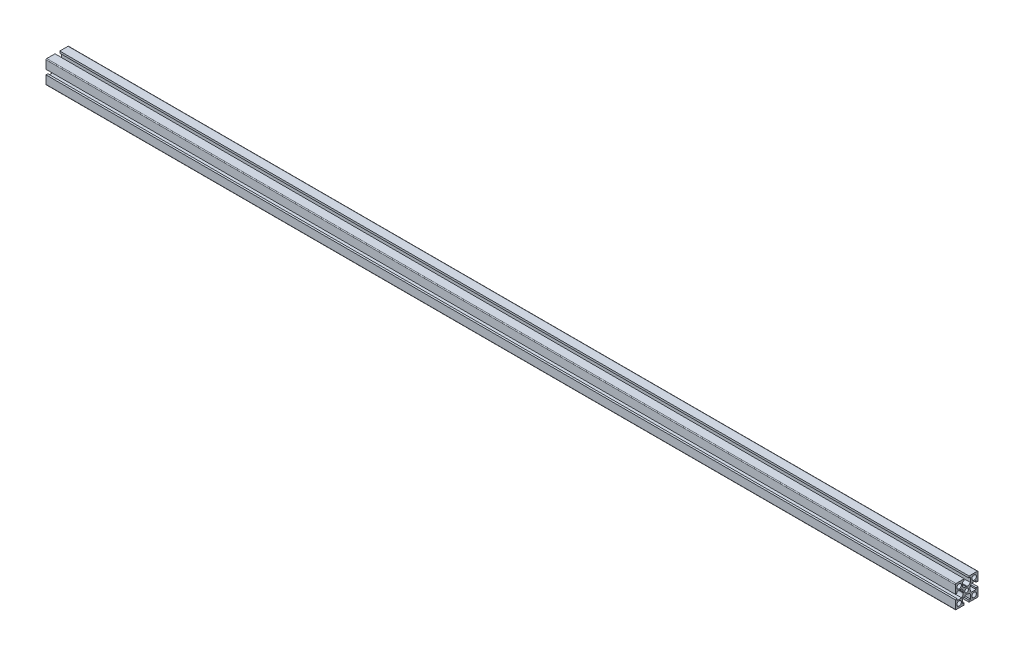
SolidWorks part; units mm, degrees
ref_plane "前视基准面" through (0, 0, 0) normal (0, 0, 1) x (1, 0, 0)
ref_plane "上视基准面" through (0, 0, 0) normal (0, 1, 0) x (1, 0, 0)
ref_plane "右视基准面" through (0, 0, 0) normal (1, 0, 0) x (0, 0, -1)
sketch "草图1" plane through (0, 0, 0) normal (0, 0, 1) x (1, 0, 0)
  line L0 (0, 0) -> (1200, 0)
  line L1 (16.5, 0) -> (-16.5, 0) construction
  dimension "D1" = 1200
other "0国耀铝型材 GY-3030国标铝型材(1)"
ref_plane "基准面1" through (0, 0, 0) normal (1, 0, 0) x (0, 1, 0)
sketch "草图11" plane through (0, 0, 0) normal (1, 0, 0) x (0, 1, 0)
  line L0 (0, 0) -> (15, 0) construction
  line L1 (0, 0) -> (0, 15) construction
  line L42 (-14, -15) -> (-3.15, -15)
  line L43 (-3.15, -15) -> (-3.15, -12.5)
  line L44 (-3.15, -12.5) -> (-5.15, -12.5)
  line L45 (-5.15, -12.5) -> (-5.15, -6.5)
  line L46 (-0.555, -4.52) -> (0, -4.2)
  line L47 (0, -4.2) -> (0.555, -4.52)
  line L48 (5.15, -6.5) -> (5.15, -12.5)
  line L49 (5.15, -12.5) -> (3.15, -12.5)
  line L50 (3.15, -12.5) -> (3.15, -15)
  line L51 (3.15, -15) -> (14, -15)
  line L52 (15, -14) -> (15, -3.15)
  line L53 (15, -3.15) -> (12.5, -3.15)
  line L54 (12.5, -3.15) -> (12.5, -5.15)
  line L55 (12.5, -5.15) -> (6.5, -5.15)
  line L56 (4.52, -0.554) -> (4.2, 0)
  line L57 (4.2, 0) -> (4.52, 0.555)
  line L58 (6.5, 5.15) -> (12.5, 5.15)
  line L59 (12.5, 5.15) -> (12.5, 3.15)
  line L60 (12.5, 3.15) -> (15, 3.15)
  line L61 (15, 3.15) -> (15, 14)
  line L62 (14, 15) -> (3.15, 15)
  line L63 (3.15, 15) -> (3.15, 12.5)
  line L64 (3.15, 12.5) -> (5.15, 12.5)
  line L65 (5.15, 12.5) -> (5.15, 6.5)
  line L66 (0.555, 4.521) -> (0, 4.2)
  line L67 (0, 4.2) -> (-0.555, 4.521)
  line L68 (-5.15, 6.5) -> (-5.15, 12.5)
  line L69 (-5.15, 12.5) -> (-3.15, 12.5)
  line L70 (-3.15, 12.5) -> (-3.15, 15)
  line L71 (-3.15, 15) -> (-14, 15)
  line L72 (-15, 14) -> (-15, 3.15)
  line L73 (-15, 3.15) -> (-12.5, 3.15)
  line L74 (-12.5, 3.15) -> (-12.5, 5.15)
  line L75 (-12.5, 5.15) -> (-6.5, 5.15)
  line L76 (-4.52, 0.555) -> (-4.2, 0)
  line L77 (-4.2, 0) -> (-4.52, -0.554)
  line L78 (-6.5, -5.15) -> (-12.5, -5.15)
  line L79 (-12.5, -5.15) -> (-12.5, -3.15)
  line L80 (-12.5, -3.15) -> (-15, -3.15)
  line L81 (-15, -3.15) -> (-15, -14)
  arc A13 (-15, -14) -> (-14, -15) centre (-14, -14) ccw
  arc A14 (-5.15, -6.5) -> (-0.555, -4.52) centre (0.0004, -12.1308) cw
  arc A15 (0.555, -4.52) -> (5.15, -6.5) centre (-0.0004, -12.1308) cw
  arc A16 (14, -15) -> (15, -14) centre (14, -14) ccw
  arc A17 (6.5, -5.15) -> (4.52, -0.554) centre (12.1308, 0.0003) cw
  arc A18 (4.52, 0.555) -> (6.5, 5.15) centre (12.1308, -0.0004) cw
  arc A19 (15, 14) -> (14, 15) centre (14, 14) ccw
  arc A20 (5.15, 6.5) -> (0.555, 4.521) centre (0.0008, 12.1318) cw
  arc A21 (-0.555, 4.521) -> (-5.15, 6.5) centre (-0.0008, 12.1318) cw
  arc A22 (-14, 15) -> (-15, 14) centre (-14, 14) ccw
  arc A23 (-6.5, 5.15) -> (-4.52, 0.555) centre (-12.1308, -0.0004) cw
  arc A24 (-4.52, -0.554) -> (-6.5, -5.15) centre (-12.1308, 0.0003) cw
  circle A25 centre (9.8, 9.9) radius 3
  circle A26 centre (9.8, -9.9) radius 3
  circle A27 centre (0, 0) radius 2.5
  circle A28 centre (-9.8, 9.9) radius 3
  circle A29 centre (-10, -9.9) radius 3
  point P0 (0, 0)
  dimension "D3" = 19.8
  dimension "D2" = 19.8
  dimension "D5" = 5
  dimension "D6" = 6
  dimension "D4" = 6.3
  dimension "D9" = 30
  dimension "D10" = 30
